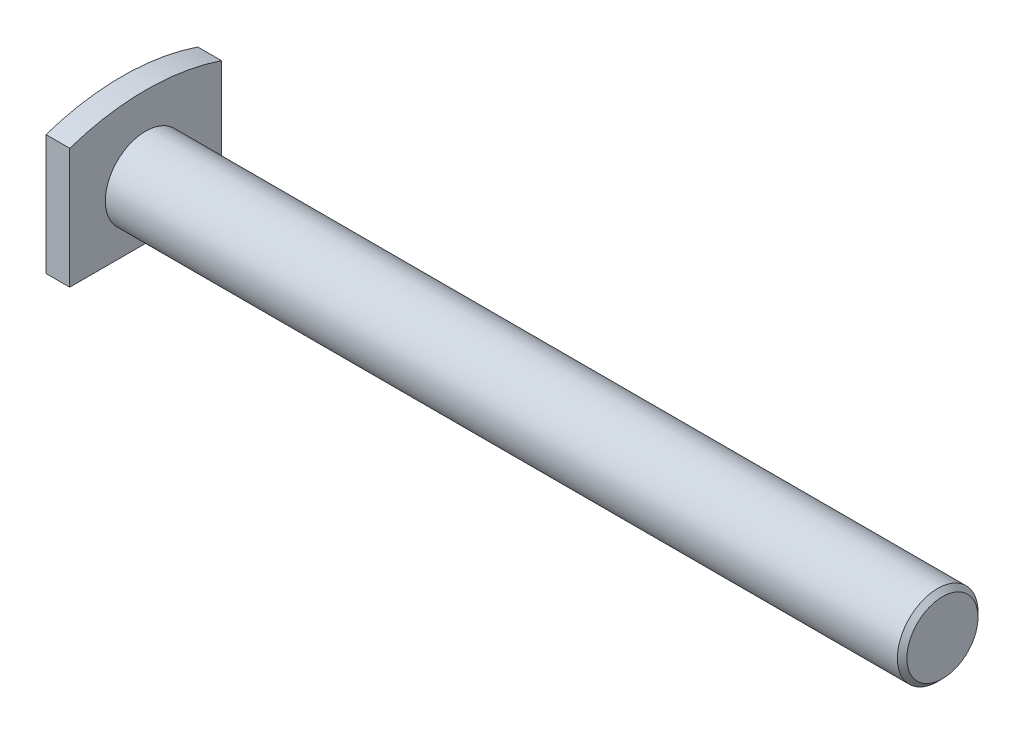
SolidWorks part; units mm, degrees
material "AL6061"
ref_plane "前视基准面" through (0, 0, 0) normal (0, 0, 1) x (1, 0, 0)
ref_plane "上视基准面" through (0, 0, 0) normal (0, 1, 0) x (1, 0, 0)
ref_plane "右视基准面" through (0, 0, 0) normal (1, 0, 0) x (0, 0, -1)
sketch "草图1" plane through (0, 0, 0) normal (0, 0, 1) x (1, 0, 0)
  line L0 (-1.1341, 0) -> (91.6893, 0) construction
  line L2 (0, 0) -> (84, 0)
  line L3 (0, 0) -> (0, -4.25)
  line L5 (84, 0) -> (84, -4.25)
  line L6 (0, -4.25) -> (84, -4.25)
  dimension "D1" = 8.5
  dimension "D2" = 84
revolve "旋转1" add sketch "草图1" angle 360 about L0
chamfer "倒角1" distance 0.5 angle 45 1 edges at (84, 0, 4.25)
sketch "草图2" plane through (0, 0, 0) normal (-1, 0, 0) x (0, 0, 1)
  line L0 (0, 5.6427) -> (0, -4.573) construction
  line L1 (-7.127, 0) -> (7.5014, 0) construction
  line L4 (-8, 6.6854) -> (-8, -6)
  line L5 (-8, -6) -> (8, -6)
  line L6 (8, 6.6854) -> (8, -6)
  arc A0 (-8, 6.6854) -> (8, 6.6854) centre (0, -17) cw
  dimension "D2" = 25
  dimension "D3" = 8
  dimension "D1" = 16
  dimension "D4" = 14
extrude "凸台-拉伸1" add sketch "草图2" along normal blind 2.5
